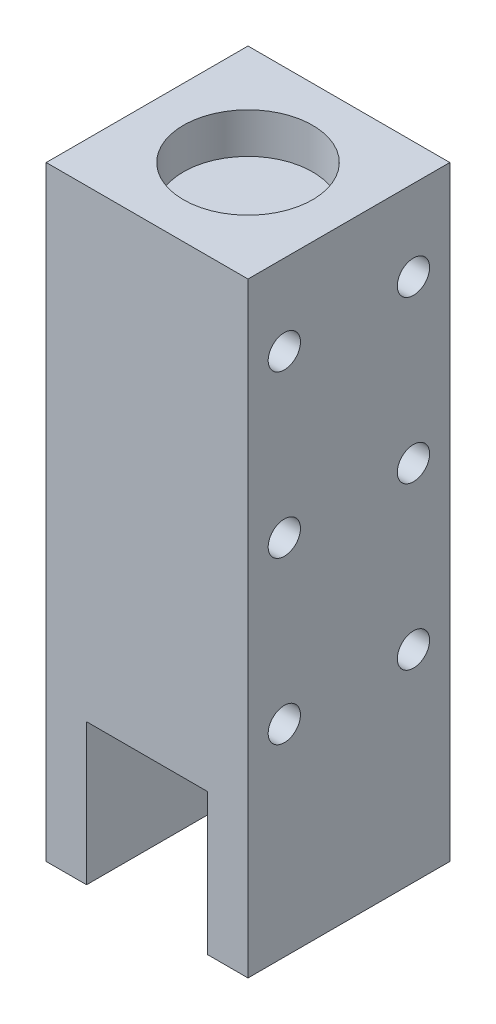
from build123d import *

# Parameters (mm, degrees)
SKETCH1_W           = 50
SKETCH1_H           = 50
BOSS_EXTRUDE2_DEPTH = 150
SKETCH2_W           = 30
SKETCH2_H           = 50
CUT_EXTRUDE1_DEPTH  = 35
SKETCH4_R           = 16
CUT_EXTRUDE2_DEPTH  = 10
SKETCH5_R           = 4
CUT_EXTRUDE3_DEPTH  = 10


with BuildPart() as part:
    # Sketch1 → Boss-Extrude2 (new body)
    with BuildSketch(Plane(origin=(0, 0, 0), x_dir=(1, 0, 0), z_dir=(0, 1, 0))):
        Rectangle(SKETCH1_W, SKETCH1_H)
    extrude(amount=BOSS_EXTRUDE2_DEPTH)

    # Sketch2 → Cut-Extrude1 (cut)
    with BuildSketch(Plane.XZ):
        Rectangle(SKETCH2_W, SKETCH2_H)
    extrude(amount=-CUT_EXTRUDE1_DEPTH, mode=Mode.SUBTRACT)

    # Sketch4 → Cut-Extrude2 (cut)
    with BuildSketch(Plane(origin=(0, 150, 0), x_dir=(1, 0, 0), z_dir=(0, 1, 0))):
        with Locations(Location((0, 0, 0), (0, 0, 270))):
            Circle(SKETCH4_R)
    extrude(amount=-CUT_EXTRUDE2_DEPTH, mode=Mode.SUBTRACT)

    # Sketch5 → Cut-Extrude3 (cut)
    with BuildSketch(Plane(origin=(25, 0, 0), x_dir=(0, 0, -1), z_dir=(1, 0, 0))):
        with Locations((-16, 130)):
            Circle(SKETCH5_R)
        with Locations((16, 130)):
            Circle(SKETCH5_R)
        with Locations((-16, 90)):
            Circle(SKETCH5_R)
        with Locations((-16, 50)):
            Circle(SKETCH5_R)
        with Locations((16, 50)):
            Circle(SKETCH5_R)
        with Locations(Location((16, 90, 0), (0, 0, 180))):
            Circle(SKETCH5_R)
    cut_extrude3 = extrude(amount=-CUT_EXTRUDE3_DEPTH, mode=Mode.SUBTRACT)

    # Mirror1: Cut-Extrude3 across plane
    add(cut_extrude3.mirror(Plane(origin=(0, 0, 0), x_dir=(0, 0, 1), z_dir=(1, 0, 0))), mode=Mode.SUBTRACT)


solid = part.part
